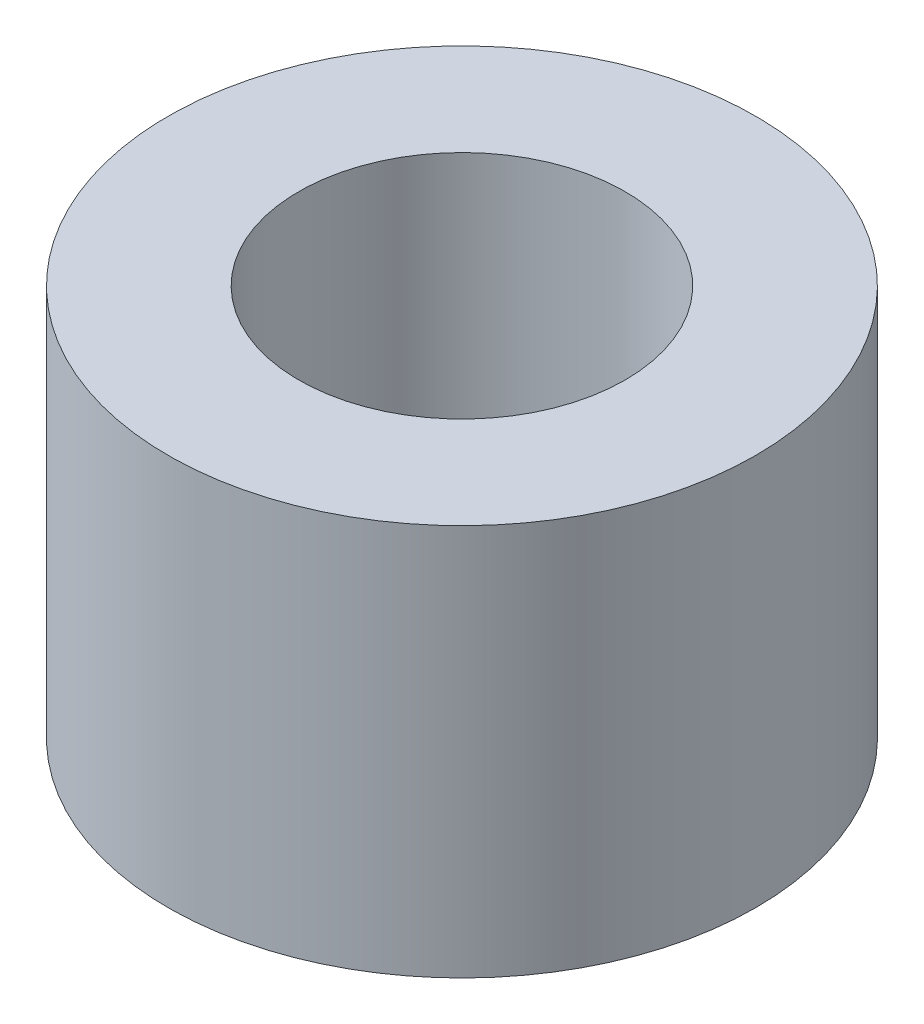
SolidWorks part; units mm, degrees
material "Plain Carbon Steel"
ref_plane "Front Plane" through (0, 0, 0) normal (0, 0, 1) x (1, 0, 0)
ref_plane "Top Plane" through (0, 0, 0) normal (0, 1, 0) x (1, 0, 0)
ref_plane "Right Plane" through (0, 0, 0) normal (1, 0, 0) x (0, 0, -1)
sketch "Sketch1" plane through (0, 0, 0) normal (0, 0, 1) x (1, 0, 0)
  line L0 (0, -483.4838) -> (0, 23690.7048) construction
  line L2 (5, 12) -> (9, 12)
  line L3 (5, 12) -> (5, 0)
  line L4 (5, 0) -> (9, 0)
  line L5 (9, 12) -> (9, 0)
  dimension "D1" = 5
  dimension "D2" = 9
  dimension "D3" = 12
revolve "Revolve1" add sketch "Sketch1" angle 360 about L0
